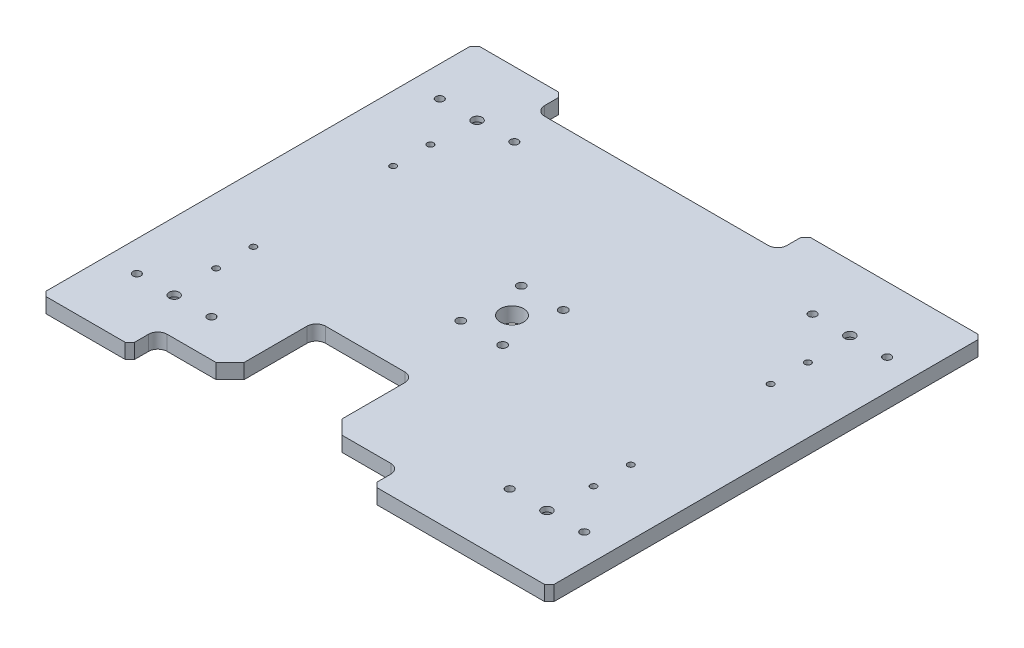
from build123d import *

# Parameters (mm, degrees)
SKETCH_1_W                     = 545
SKETCH_1_H                     = 465
EXTRUDE_1_DEPTH                = 8
SKETCH_2_W                     = 260
SKETCH_2_H                     = 30
CUT_EXTRUDE_1_DEPTH            = 16
SKETCH_3_W                     = 105
SKETCH_3_H                     = 122.5
CUT_EXTRUDE_2_DEPTH            = 359.564499079
HOLE_WIZARD_M8_2_D             = 6.8
MIRROR_3_COPY_1_D              = 6.8
CHAMFER_1_SIZE                 = 15
FILLET_1_R                     = 10
HOLE_WIZARD_9_0_9_1_D          = 9
HOLE_WIZARD_M10_1_D            = 11
HOLE_WIZARD_M10_1_DEPTH        = 24.5
HOLE_WIZARD_M10_1_CBORE_D      = 18
HOLE_WIZARD_M10_1_CBORE_DEPTH  = 10.6
HOLE_WIZARD_M10_1_TIP          = 3.304733405
CHAMFER_2_SIZE                 = 5
HOLE_WIZARD_M10_1_2_AT_2_COUNT = 2
HOLE_WIZARD_M10_1_2_AT_2_PITCH = 80
SKETCH_17_R                    = 12.5
CUT_EXTRUDE_10_DEPTH           = 359.564499079


with BuildPart() as part:
    # 草图1 → 凸台-拉伸1 (new, symmetric)
    with BuildSketch(Plane(origin=(0, 0, 0), x_dir=(1, 0, 0), z_dir=(0, 1, 0))):
        Rectangle(SKETCH_1_W, SKETCH_1_H)
    extrude(amount=EXTRUDE_1_DEPTH, both=True)

    # 草图2 → 切除-拉伸1 (cut)
    with BuildSketch(Plane(origin=(0, 8, 0), x_dir=(1, 0, 0), z_dir=(0, 1, 0))):
        with Locations((-47.5, 217.5)):
            Rectangle(SKETCH_2_W, SKETCH_2_H)
    cut_extrude_1 = extrude(amount=-CUT_EXTRUDE_1_DEPTH, mode=Mode.SUBTRACT)

    # 镜向1: 切除-拉伸1 across plane
    add(cut_extrude_1.mirror(Plane.XY), mode=Mode.SUBTRACT)

    # 草图3 → 切除-拉伸2 (cut, through all)
    with BuildSketch(Plane(origin=(0, 8, 0), x_dir=(1, 0, 0), z_dir=(0, 1, 0))):
        with Locations((-47.5, -171.25)):
            Rectangle(SKETCH_3_W, SKETCH_3_H)
    extrude(amount=-CUT_EXTRUDE_2_DEPTH, mode=Mode.SUBTRACT)

    # M8 螺纹孔2 (through all)
    with Locations(Plane(origin=(0, 8, 0), x_dir=(1, 0, 0), z_dir=(0, 1, 0))):
        with Locations((202.5, -115), (202.5, -75)):
            hole_wizard_m8_2 = Hole(HOLE_WIZARD_M8_2_D / 2)

    # 镜向2: M8 螺纹孔2 across plane
    add(hole_wizard_m8_2.mirror(Plane(origin=(0, 0, 0), x_dir=(0, 0, 1), z_dir=(1, 0, 0))), mode=Mode.SUBTRACT)

    # 镜向3: M8 螺纹孔2 across plane
    add(hole_wizard_m8_2.mirror(Plane.XY), mode=Mode.SUBTRACT)

    # 镜向3 copy 1 (through all)
    with Locations(Plane(origin=(0, 8, 0), x_dir=(-1, 0, 0), z_dir=(0, 1, 0))):
        with Locations((202.5, -115), (202.5, -75)):
            Hole(MIRROR_3_COPY_1_D / 2)

    # 倒角1
    chamfer_1_edges = [part.edges().sort_by_distance(p)[0] for p in [
        (5, 0, 202.5),
        (-100, 0, 202.5),
    ]]
    chamfer(chamfer_1_edges, length=CHAMFER_1_SIZE)

    # 圆角1
    fillet_1_edges = [part.edges().sort_by_distance(p)[0] for p in [
        (-177.5, 0, -202.5),
        (82.5, 0, -202.5),
        (-177.5, 0, 202.5),
        (82.5, 0, 202.5),
        (-100, 0, 110),
        (5, 0, 110),
    ]]
    fillet(fillet_1_edges, radius=FILLET_1_R)

    # Ø9.0 (9) 直径孔1 (through all)
    with Locations(Plane(origin=(0, 8, 0), x_dir=(1, 0, 0), z_dir=(0, 1, 0))):
        with Locations((22.5, -32.5), (-22.5, -32.5), (-22.5, 32.5), (22.5, 32.5)):
            Hole(HOLE_WIZARD_9_0_9_1_D / 2)

    # Hole Wizard M10 _1
    with Locations(Plane.XZ.offset(8)):
        with Locations((-200, -162.5), (200, -162.5), (-200, 162.5), (200, 162.5)):
            CounterBoreHole(HOLE_WIZARD_M10_1_D / 2, HOLE_WIZARD_M10_1_CBORE_D / 2, HOLE_WIZARD_M10_1_CBORE_DEPTH, depth=HOLE_WIZARD_M10_1_DEPTH)
            with Locations((0, 0, -(HOLE_WIZARD_M10_1_DEPTH + HOLE_WIZARD_M10_1_TIP / 2))):  # 118° drill point
                Cone(0, HOLE_WIZARD_M10_1_D / 2, HOLE_WIZARD_M10_1_TIP, mode=Mode.SUBTRACT)

    # 倒角2
    chamfer_2_edges = [part.edges().sort_by_distance(p)[0] for p in [
        (-177.5, 0, -232.5),
        (82.5, 0, -232.5),
        (-177.5, 0, 232.5),
        (82.5, 0, 232.5),
        (272.5, 0, 232.5),
        (-272.5, 0, 232.5),
        (-272.5, 0, -232.5),
        (272.5, 0, -232.5),
    ]]
    chamfer(chamfer_2_edges, length=CHAMFER_2_SIZE)

    # 草图15 → Hole Wizard M10 _1 2 (revolve, cut)
    with BuildSketch(Plane(origin=(-240, 8, 162.5), x_dir=(0, 0, 1), z_dir=(1, 0, 0))):
        Polygon((0, 0), (0, 27.053657631), (4.25, 24.5), (4.25, 0), align=None)
    hole_wizard_m10_1_2 = revolve(axis=Axis((-240, 14.35, 162.5), (0, -1, 0)), mode=Mode.SUBTRACT)

    # Hole Wizard M10 _1 2 at 2: Hole Wizard M10 _1 2 ×2
    with Locations(*[(i * HOLE_WIZARD_M10_1_2_AT_2_PITCH, 0, 0) for i in range(1, HOLE_WIZARD_M10_1_2_AT_2_COUNT)]):
        add(hole_wizard_m10_1_2, mode=Mode.SUBTRACT)

    # 镜向4: Hole Wizard M10 _1 2 across plane
    add(hole_wizard_m10_1_2.mirror(Plane.XY), mode=Mode.SUBTRACT)

    # 镜向4 copy 1 sketch → 镜向4 copy 1 (revolve, cut)
    with BuildSketch(Plane(origin=(-160, 8, -162.5), x_dir=(0, 0, -1), z_dir=(1, 0, 0))):
        Polygon((0, 0), (0, -27.053657631), (4.25, -24.5), (4.25, 0), align=None)
    revolve(axis=Axis((-160, 14.35, -162.5), (0, 1, 0)), mode=Mode.SUBTRACT)

    # 镜向5: Hole Wizard M10 _1 2 across plane
    add(hole_wizard_m10_1_2.mirror(Plane(origin=(0, 0, 0), x_dir=(0, 0, 1), z_dir=(1, 0, 0))), mode=Mode.SUBTRACT)

    # 镜向5 copy 1 sketch → 镜向5 copy 1 (revolve, cut)
    with BuildSketch(Plane(origin=(160, 8, 162.5), x_dir=(0, 0, 1), z_dir=(-1, 0, 0))):
        Polygon((0, 0), (0, -27.053657631), (4.25, -24.5), (4.25, 0), align=None)
    revolve(axis=Axis((160, 14.35, 162.5), (0, 1, 0)), mode=Mode.SUBTRACT)

    # 镜向5 copy 2 sketch → 镜向5 copy 2 (revolve, cut)
    with BuildSketch(Plane(origin=(240, 8, -162.5), x_dir=(0, 0, -1), z_dir=(-1, 0, 0))):
        Polygon((0, 0), (0, 27.053657631), (4.25, 24.5), (4.25, 0), align=None)
    revolve(axis=Axis((240, 14.35, -162.5), (0, -1, 0)), mode=Mode.SUBTRACT)

    # 镜向5 copy 3 sketch → 镜向5 copy 3 (revolve, cut)
    with BuildSketch(Plane(origin=(160, 8, -162.5), x_dir=(0, 0, -1), z_dir=(-1, 0, 0))):
        Polygon((0, 0), (0, 27.053657631), (4.25, 24.5), (4.25, 0), align=None)
    revolve(axis=Axis((160, 14.35, -162.5), (0, -1, 0)), mode=Mode.SUBTRACT)

    # 草图17 → 切除-拉伸10 (cut, through all)
    with BuildSketch(Plane(origin=(0, 8, 0), x_dir=(1, 0, 0), z_dir=(0, 1, 0))):
        with Locations(Location((0, 0, 0), (0, 0, 270))):
            Circle(SKETCH_17_R)
    extrude(amount=-CUT_EXTRUDE_10_DEPTH, mode=Mode.SUBTRACT)


solid = part.part
